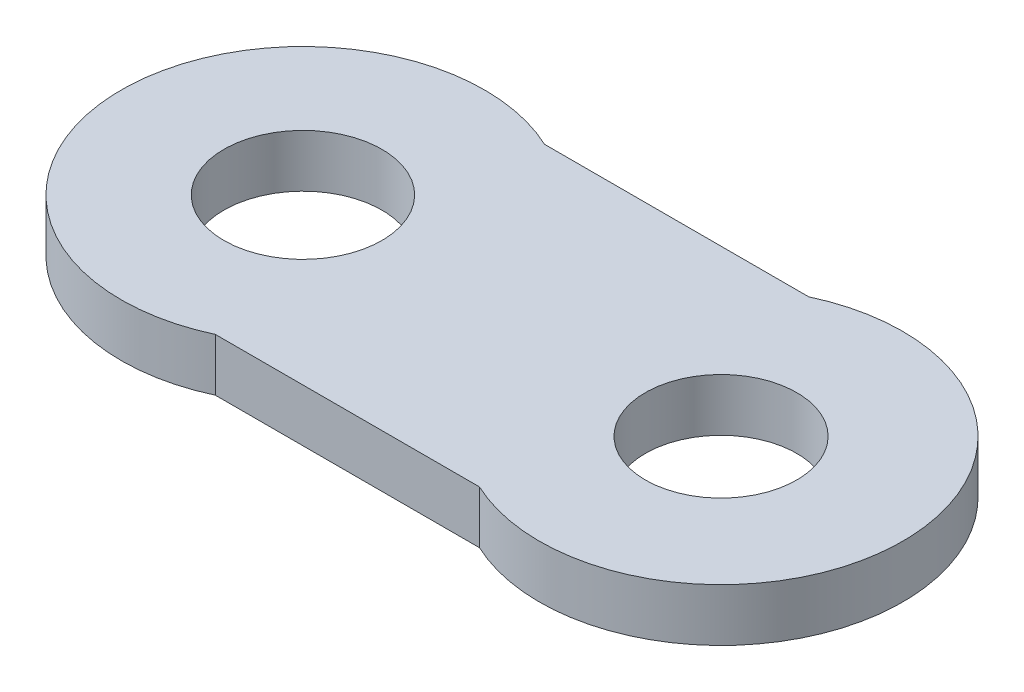
from build123d import *

# Parameters (mm, degrees)
SKETCH_1_R      = 1.2
SKETCH_1_R_2    = 1.15
EXTRUDE_1_DEPTH = 0.8


with BuildPart() as part:
    # 草图1 → 凸台-拉伸1 (new body)
    with BuildSketch(Plane(origin=(0, 0, 0), x_dir=(1, 0, 0), z_dir=(0, 1, 0))):
        with BuildLine():
            Line((-1.079891697, 2.5), (2.931219678, 2.5))
            ThreePointArc((2.931219678, 2.5), (6.860663991, 0), (2.931219678, -2.5))
            Line((2.931219678, -2.5), (-1.079891697, -2.5))
            ThreePointArc((-1.079891697, -2.5), (-5.009336009, 0), (-1.079891697, 2.5))
        make_face()
        with Locations(Location((-2.249336009, 0, 0), (0, 0, 270))):
            Circle(SKETCH_1_R, mode=Mode.SUBTRACT)
        with Locations(Location((4.100663991, 0, 0), (0, 0, 270))):
            Circle(SKETCH_1_R_2, mode=Mode.SUBTRACT)
    extrude(amount=EXTRUDE_1_DEPTH)


solid = part.part
